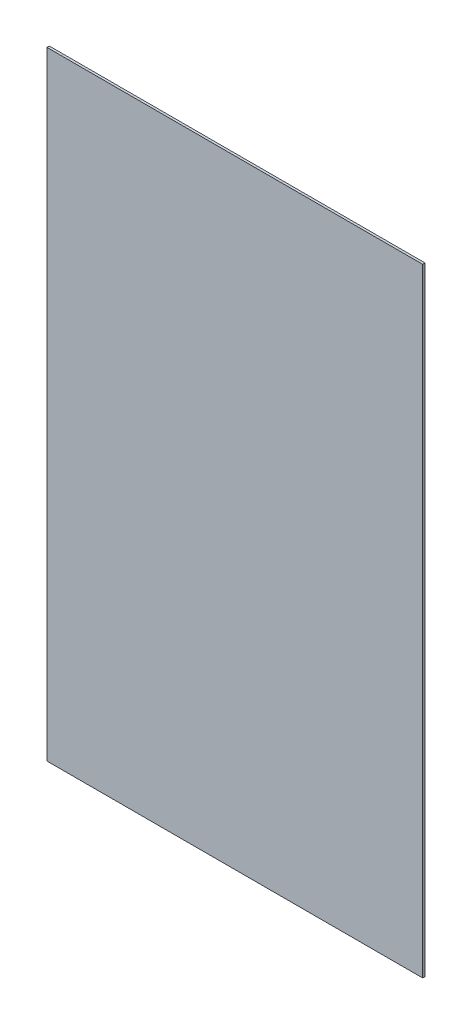
from build123d import *

# Parameters (mm, degrees)
SKETCH_1_W      = 794
SKETCH_1_H      = 1306
EXTRUDE_1_DEPTH = 5


with BuildPart() as part:
    # 草图1 → 凸台-拉伸1 (new body)
    with BuildSketch(Plane.XY):
        Rectangle(SKETCH_1_W, SKETCH_1_H)
    extrude(amount=EXTRUDE_1_DEPTH)


solid = part.part
